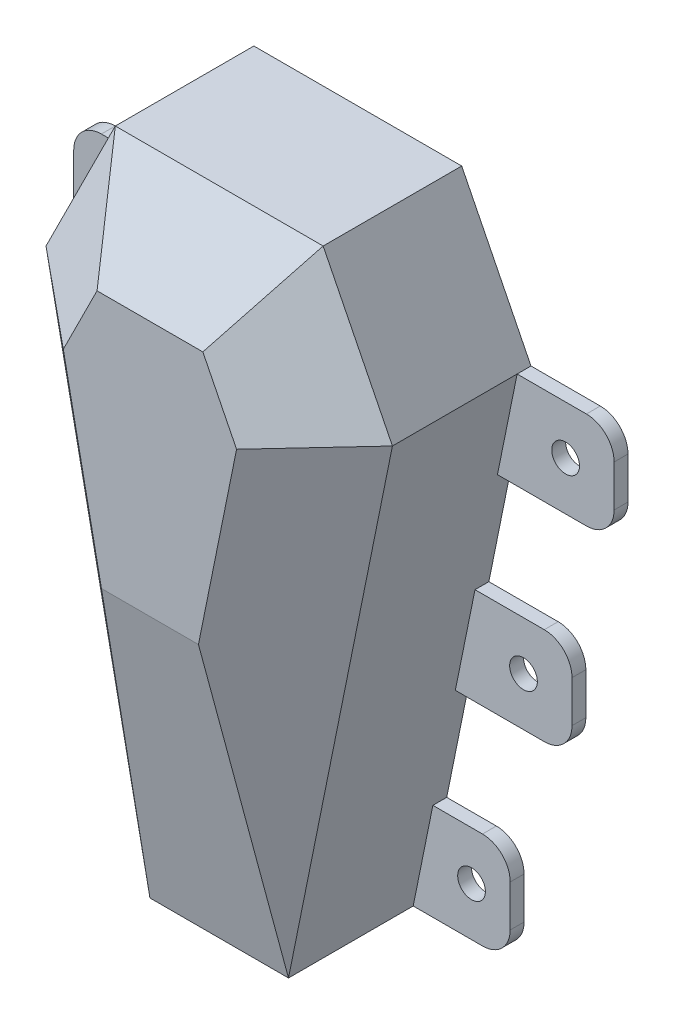
from build123d import *

# Parameters (mm, degrees)
BOSS_EXTRUDE1_DEPTH  = 50
BOSS_EXTRUDE1_TAPER  = 50
CUT_EXTRUDE2_DEPTH   = 438
SHELL1_T             = -5
BOSS_EXTRUDE2_DEPTH  = 100
BOSS_EXTRUDE3_DEPTH  = 5
SKETCH9_R            = 10
BOSS_EXTRUDE4_DEPTH  = 10
FILLET1_R            = 20
FILLET2_R            = 20
FILLET3_R            = 20
SKETCH19_R           = 10
BOSS_EXTRUDE6_DEPTH  = 50
SKETCH35_R           = 10
BOSS_EXTRUDE7_DEPTH  = 50
SKETCH36_R           = 10
BOSS_EXTRUDE8_DEPTH  = 50
SKETCH37_R           = 10
BOSS_EXTRUDE9_DEPTH  = 50
SKETCH38_R           = 10
BOSS_EXTRUDE10_DEPTH = 50
SKETCH39_R           = 10
BOSS_EXTRUDE11_DEPTH = 50
SKETCH45_R           = 10
CUT_EXTRUDE3_DEPTH   = 50
CUT_EXTRUDE4_DEPTH   = 50
CUT_EXTRUDE5_DEPTH   = 50
CUT_EXTRUDE6_DEPTH   = 50
CUT_EXTRUDE7_DEPTH   = 50
CUT_EXTRUDE8_DEPTH   = 50


with BuildPart() as part:
    # Sketch2 → Boss-Extrude1 (new body)
    with BuildSketch(Plane.XY):
        Polygon((-50, 0), (50, 0), (125, 370), (75, 470), (-75, 470), (-125, 370), align=None)
    extrude(amount=BOSS_EXTRUDE1_DEPTH, taper=BOSS_EXTRUDE1_TAPER)

    # Sketch5 → Cut-Extrude2 (cut, symmetric)
    with BuildSketch(Plane(origin=(0, 0, 0), x_dir=(0, 0, -1), z_dir=(1, 0, 0))):
        Polygon((-50, 225.964141046), (0, 0), (-90.655287841, 0), align=None)
    extrude(amount=CUT_EXTRUDE2_DEPTH, both=True, mode=Mode.SUBTRACT)

    # Shell1
    shell1_openings = [part.faces().sort_by_distance(p)[0] for p in [
        (0, 259.665683382, 0),
    ]]
    offset(amount=SHELL1_T, openings=shell1_openings, kind=Kind.INTERSECTION)

    # Sketch6 → Boss-Extrude2 (add)
    with BuildSketch(Plane(origin=(0, 0, 0), x_dir=(-1, 0, 0), z_dir=(0, 0, -1))):
        Polygon((50, 0), (125, 370), (75, 470), (-75, 470), (-125, 370), (-50, 0), align=None)
        Polygon((-116.843969267, 368.91854031), (-70.192548989, 462.221380866), (70.192548989, 462.221380866), (116.843969267, 368.91854031), (46.754330446, 23.142988795), (-46.754330446, 23.142988795), align=None, mode=Mode.SUBTRACT)
    extrude(amount=BOSS_EXTRUDE2_DEPTH)

    # Sketch7 → Boss-Extrude3 (add)
    with BuildSketch(Plane(origin=(0, 0, -100), x_dir=(-1, 0, 0), z_dir=(0, 0, -1))):
        Polygon((-46.754330446, 23.142988795), (-116.843969267, 368.91854031), (-70.192548989, 462.221380866), (70.192548989, 462.221380866), (116.843969267, 368.91854031), (46.754330446, 23.142988795), align=None)
    extrude(amount=-BOSS_EXTRUDE3_DEPTH)

    # Sketch9 → Boss-Extrude4 (add)
    # profile 1 of 3: a face of its own
    with BuildSketch(Plane.XY.offset(-50)):
        Polygon((125, 370), (110.810810811, 300), (195, 300), (195, 370), align=None)
        with Locations((160, 335)):
            Circle(SKETCH9_R, mode=Mode.SUBTRACT)
    # profile 2 of 3: a face of its own
    with BuildSketch(Plane.XY.offset(-50)):
        Polygon((94.594594595, 220), (80.405405405, 150), (164.594594595, 150), (164.594594595, 220), align=None)
        with Locations((129.594594595, 185)):
            Circle(SKETCH9_R, mode=Mode.SUBTRACT)
    # profile 3 of 3: a face of its own
    with BuildSketch(Plane.XY.offset(-50)):
        Polygon((64.189189189, 70), (50, 0), (120, 0), (120, 70), align=None)
        with Locations((92.094594595, 35)):
            Circle(SKETCH9_R, mode=Mode.SUBTRACT)
    boss_extrude4 = extrude(amount=BOSS_EXTRUDE4_DEPTH)

    # Fillet1
    fillet1_edges = [part.edges().sort_by_distance(p)[0] for p in [
        (195, 300, -45),
        (195, 370, -45),
    ]]
    fillet(fillet1_edges, radius=FILLET1_R)

    # Fillet2
    fillet2_edges = [part.edges().sort_by_distance(p)[0] for p in [
        (164.594594595, 150, -45),
        (164.594594595, 220, -45),
        (120, 0, -45),
        (120, 70, -45),
    ]]
    fillet(fillet2_edges, radius=FILLET2_R)

    # Mirror1: Boss-Extrude4 across plane
    add(boss_extrude4.mirror(Plane(origin=(0, 0, 0), x_dir=(0, 0, 1), z_dir=(1, 0, 0))))

    # Fillet3
    fillet3_edges = [part.edges().sort_by_distance(p)[0] for p in [
        (-195, 300, -45),
        (-195, 370, -45),
        (-164.594594595, 150, -45),
        (-164.594594595, 220, -45),
        (-120, 70, -45),
        (-120, 0, -45),
    ]]
    fillet(fillet3_edges, radius=FILLET3_R)

    # Sketch19 → Boss-Extrude6 (add)
    with BuildSketch(Plane(origin=(0, 0, -50), x_dir=(-1, 0, 0), z_dir=(0, 0, -1))):
        with BuildLine():
            Line((94.594594595, 220), (80.405405405, 150))
            Line((80.405405405, 150), (144.594594595, 150))
            ThreePointArc((144.594594595, 150), (158.736730218, 155.857864376), (164.594594595, 170))
            Line((164.594594595, 170), (164.594594595, 200))
            ThreePointArc((164.594594595, 200), (158.736730218, 214.142135624), (144.594594595, 220))
            Line((144.594594595, 220), (94.594594595, 220))
        make_face()
        with Locations((129.594594595, 185)):
            Circle(SKETCH19_R, mode=Mode.SUBTRACT)
    extrude(amount=BOSS_EXTRUDE6_DEPTH)

    # Sketch35 → Boss-Extrude7 (add)
    with BuildSketch(Plane(origin=(0, 0, -50), x_dir=(-1, 0, 0), z_dir=(0, 0, -1))):
        with BuildLine():
            Line((110.810810811, 300), (175, 300))
            ThreePointArc((175, 300), (189.142135624, 305.857864376), (195, 320))
            Line((195, 320), (195, 350))
            ThreePointArc((195, 350), (189.142135624, 364.142135624), (175, 370))
            Line((175, 370), (125, 370))
            Line((125, 370), (110.810810811, 300))
        make_face()
        with Locations((160, 335)):
            Circle(SKETCH35_R, mode=Mode.SUBTRACT)
    extrude(amount=BOSS_EXTRUDE7_DEPTH)

    # Sketch36 → Boss-Extrude8 (add)
    with BuildSketch(Plane(origin=(0, 0, -50), x_dir=(-1, 0, 0), z_dir=(0, 0, -1))):
        with BuildLine():
            Line((64.189189189, 70), (50, 0))
            Line((50, 0), (100, 0))
            ThreePointArc((100, 0), (114.142135624, 5.857864376), (120, 20))
            Line((120, 20), (120, 50))
            ThreePointArc((120, 50), (114.142135624, 64.142135624), (100, 70))
            Line((100, 70), (64.189189189, 70))
        make_face()
        with Locations((92.094594595, 35)):
            Circle(SKETCH36_R, mode=Mode.SUBTRACT)
    extrude(amount=BOSS_EXTRUDE8_DEPTH)

    # Sketch37 → Boss-Extrude9 (add)
    with BuildSketch(Plane(origin=(0, 0, -50), x_dir=(-1, 0, 0), z_dir=(0, 0, -1))):
        with BuildLine():
            Line((-100, 70), (-64.189189189, 70))
            Line((-64.189189189, 70), (-50, 0))
            Line((-50, 0), (-100, 0))
            ThreePointArc((-100, 0), (-114.142135624, 5.857864376), (-120, 20))
            Line((-120, 20), (-120, 50))
            ThreePointArc((-120, 50), (-114.142135624, 64.142135624), (-100, 70))
        make_face()
        with Locations((-92.094594595, 35)):
            Circle(SKETCH37_R, mode=Mode.SUBTRACT)
    extrude(amount=BOSS_EXTRUDE9_DEPTH)

    # Sketch38 → Boss-Extrude10 (add)
    with BuildSketch(Plane(origin=(0, 0, -50), x_dir=(-1, 0, 0), z_dir=(0, 0, -1))):
        with BuildLine():
            Line((-144.594594595, 220), (-94.594594595, 220))
            Line((-94.594594595, 220), (-80.405405405, 150))
            Line((-80.405405405, 150), (-144.594594595, 150))
            ThreePointArc((-144.594594595, 150), (-158.736730218, 155.857864376), (-164.594594595, 170))
            Line((-164.594594595, 170), (-164.594594595, 200))
            ThreePointArc((-164.594594595, 200), (-158.736730218, 214.142135624), (-144.594594595, 220))
        make_face()
        with Locations((-129.594594595, 185)):
            Circle(SKETCH38_R, mode=Mode.SUBTRACT)
    extrude(amount=BOSS_EXTRUDE10_DEPTH)

    # Sketch39 → Boss-Extrude11 (add)
    with BuildSketch(Plane(origin=(0, 0, -50), x_dir=(-1, 0, 0), z_dir=(0, 0, -1))):
        with BuildLine():
            Line((-175, 370), (-125, 370))
            Line((-125, 370), (-110.810810811, 300))
            Line((-110.810810811, 300), (-175, 300))
            ThreePointArc((-175, 300), (-189.142135624, 305.857864376), (-195, 320))
            Line((-195, 320), (-195, 350))
            ThreePointArc((-195, 350), (-189.142135624, 364.142135624), (-175, 370))
        make_face()
        with Locations((-160, 335)):
            Circle(SKETCH39_R, mode=Mode.SUBTRACT)
    extrude(amount=BOSS_EXTRUDE11_DEPTH)

    # Sketch45 → Cut-Extrude3 (cut)
    with BuildSketch(Plane.XY.offset(-40)):
        with BuildLine():
            Line((-175, 370), (-125, 370))
            Line((-125, 370), (-110.810810811, 300))
            Line((-110.810810811, 300), (-175, 300))
            ThreePointArc((-175, 300), (-189.142135624, 305.857864376), (-195, 320))
            Line((-195, 320), (-195, 350))
            ThreePointArc((-195, 350), (-189.142135624, 364.142135624), (-175, 370))
        make_face()
        with Locations(Location((-160, 335, 0), (0, 0, 180))):
            Circle(SKETCH45_R, mode=Mode.SUBTRACT)
    extrude(amount=-CUT_EXTRUDE3_DEPTH, mode=Mode.SUBTRACT)

    # Sketch46 → Cut-Extrude4 (cut)
    with BuildSketch(Plane.XY.offset(-40)):
        with BuildLine():
            Line((-144.594594595, 220), (-94.594594595, 220))
            Line((-94.594594595, 220), (-80.405405405, 150))
            Line((-80.405405405, 150), (-144.594594595, 150))
            ThreePointArc((-144.594594595, 150), (-158.736730218, 155.857864376), (-164.594594595, 170))
            Line((-164.594594595, 170), (-164.594594595, 200))
            ThreePointArc((-164.594594595, 200), (-158.736730218, 214.142135624), (-144.594594595, 220))
        make_face()
    extrude(amount=-CUT_EXTRUDE4_DEPTH, mode=Mode.SUBTRACT)

    # Sketch47 → Cut-Extrude5 (cut)
    with BuildSketch(Plane.XY.offset(-40)):
        with BuildLine():
            Line((-100, 70), (-64.189189189, 70))
            Line((-64.189189189, 70), (-50, 0))
            Line((-50, 0), (-100, 0))
            ThreePointArc((-100, 0), (-114.142135624, 5.857864376), (-120, 20))
            Line((-120, 20), (-120, 50))
            ThreePointArc((-120, 50), (-114.142135624, 64.142135624), (-100, 70))
        make_face()
    extrude(amount=-CUT_EXTRUDE5_DEPTH, mode=Mode.SUBTRACT)

    # Sketch49 → Cut-Extrude6 (cut)
    with BuildSketch(Plane.XY.offset(-40)):
        with BuildLine():
            Line((125, 370), (175, 370))
            ThreePointArc((175, 370), (189.142135624, 364.142135624), (195, 350))
            Line((195, 350), (195, 320))
            ThreePointArc((195, 320), (189.142135624, 305.857864376), (175, 300))
            Line((175, 300), (110.810810811, 300))
            Line((110.810810811, 300), (125, 370))
        make_face()
    extrude(amount=-CUT_EXTRUDE6_DEPTH, mode=Mode.SUBTRACT)

    # Sketch50 → Cut-Extrude7 (cut)
    with BuildSketch(Plane.XY.offset(-40)):
        with BuildLine():
            Line((94.594594595, 220), (144.594594595, 220))
            ThreePointArc((144.594594595, 220), (158.736730218, 214.142135624), (164.594594595, 200))
            Line((164.594594595, 200), (164.594594595, 170))
            ThreePointArc((164.594594595, 170), (158.736730218, 155.857864376), (144.594594595, 150))
            Line((144.594594595, 150), (80.405405405, 150))
            Line((80.405405405, 150), (94.594594595, 220))
        make_face()
    extrude(amount=-CUT_EXTRUDE7_DEPTH, mode=Mode.SUBTRACT)

    # Sketch51 → Cut-Extrude8 (cut)
    with BuildSketch(Plane.XY.offset(-40)):
        with BuildLine():
            Line((100, 70), (64.189189189, 70))
            Line((64.189189189, 70), (50, 0))
            Line((50, 0), (100, 0))
            ThreePointArc((100, 0), (114.142135624, 5.857864376), (120, 20))
            Line((120, 20), (120, 50))
            ThreePointArc((120, 50), (114.142135624, 64.142135624), (100, 70))
        make_face()
    extrude(amount=-CUT_EXTRUDE8_DEPTH, mode=Mode.SUBTRACT)


solid = part.part
